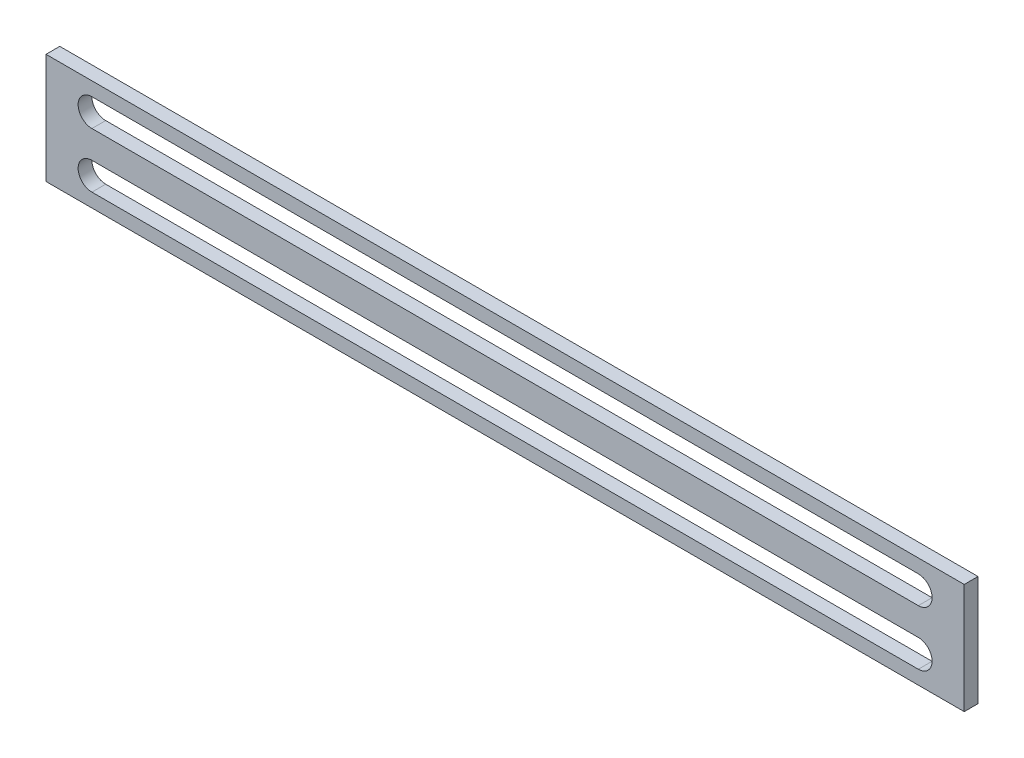
SolidWorks part; units mm, degrees
ref_plane "前视基准面" through (0, 0, 0) normal (0, 0, 1) x (1, 0, 0)
ref_plane "上视基准面" through (0, 0, 0) normal (0, 1, 0) x (1, 0, 0)
ref_plane "右视基准面" through (0, 0, 0) normal (1, 0, 0) x (0, 0, -1)
sketch "草图1" plane through (0, 0, 0) normal (0, 0, 1) x (1, 0, 0)
  line L0 (-45, 3) -> (45, 3) construction
  line L1 (50, 6) -> (-50, 6)
  line L2 (50, 6) -> (50, -6)
  line L3 (50, -6) -> (-50, -6)
  line L4 (-50, 6) -> (-50, -6)
  line L5 (50, 6) -> (-50, -6) construction
  line L6 (50, -6) -> (-50, 6) construction
  line L7 (-45, 4.5) -> (45, 4.5)
  line L8 (-45, 1.5) -> (45, 1.5)
  line L9 (-52.8458, 0) -> (68.8809, 0) construction
  line L10 (-45, -3) -> (45, -3) construction
  line L11 (-45, -4.5) -> (45, -4.5)
  line L12 (-45, -1.5) -> (45, -1.5)
  arc A0 (-45, 4.5) -> (-45, 1.5) centre (-45, 3) ccw
  arc A1 (45, 1.5) -> (45, 4.5) centre (45, 3) ccw
  arc A2 (-45, -4.5) -> (-45, -1.5) centre (-45, -3) cw
  arc A3 (45, -1.5) -> (45, -4.5) centre (45, -3) cw
  point P0 (0, 0)
  point P8 (0, 3)
  point P17 (0, -3)
  dimension "D3" = 1.5
  dimension "D1" = 12
  dimension "D2" = 100
  dimension "D4" = 90
  dimension "D5" = 3
  dimension "D6" = 5
extrude "凸台-拉伸1" add sketch "草图1" along normal blind 1.5
